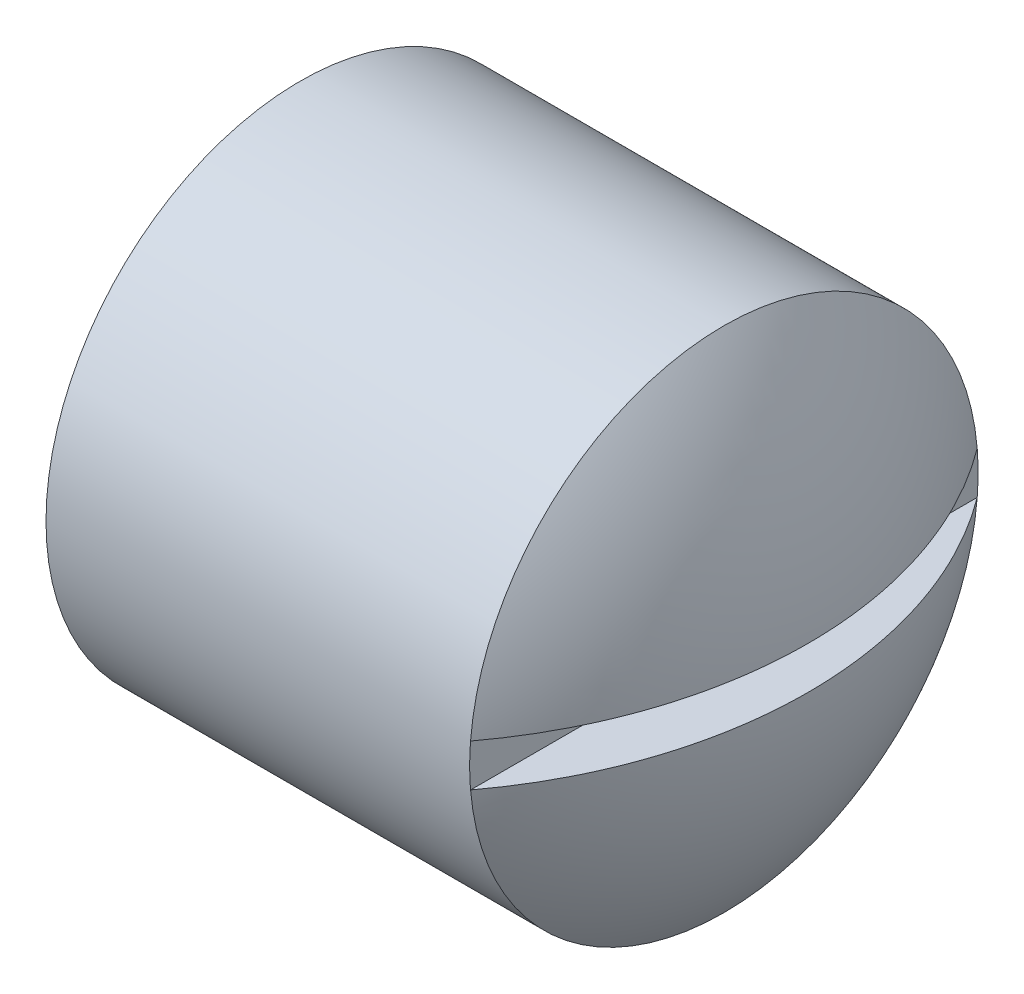
from build123d import *

# Parameters (mm, degrees)
CUT_EXTRUDE1_DEPTH      = 30.393876913
CUT_EXTRUDE1_DEPTH_BACK = 30.393876913
SKETCH2_W               = 8
SKETCH2_H               = 2


with BuildPart() as part:
    # Sketch1 → Revolve1 (revolve)
    with BuildSketch(Plane.XY, mode=Mode.PRIVATE) as revolve1_sk:
        with BuildLine():
            Line((0, 0), (0, 12))
            Line((0, 12), (20, 12))
            ThreePointArc((20, 12), (22.973665961, 6.32455532), (24, 0))
            Line((24, 0), (0, 0))
        make_face()
    revolve(revolve1_sk.sketch.rotate(Axis((0, 0, 0), (1, 0, 0)), 90), axis=Axis((0, 0, 0), (1, 0, 0)))

    # Sketch2 → Cut-Extrude1 (cut, two sides: drawn at the far end of the back side and taken through both)
    with BuildSketch(Plane.XY.offset(-CUT_EXTRUDE1_DEPTH_BACK)):
        with Locations((24, 0)):
            Rectangle(SKETCH2_W, SKETCH2_H)
    extrude(amount=CUT_EXTRUDE1_DEPTH + CUT_EXTRUDE1_DEPTH_BACK, mode=Mode.SUBTRACT)


solid = part.part
